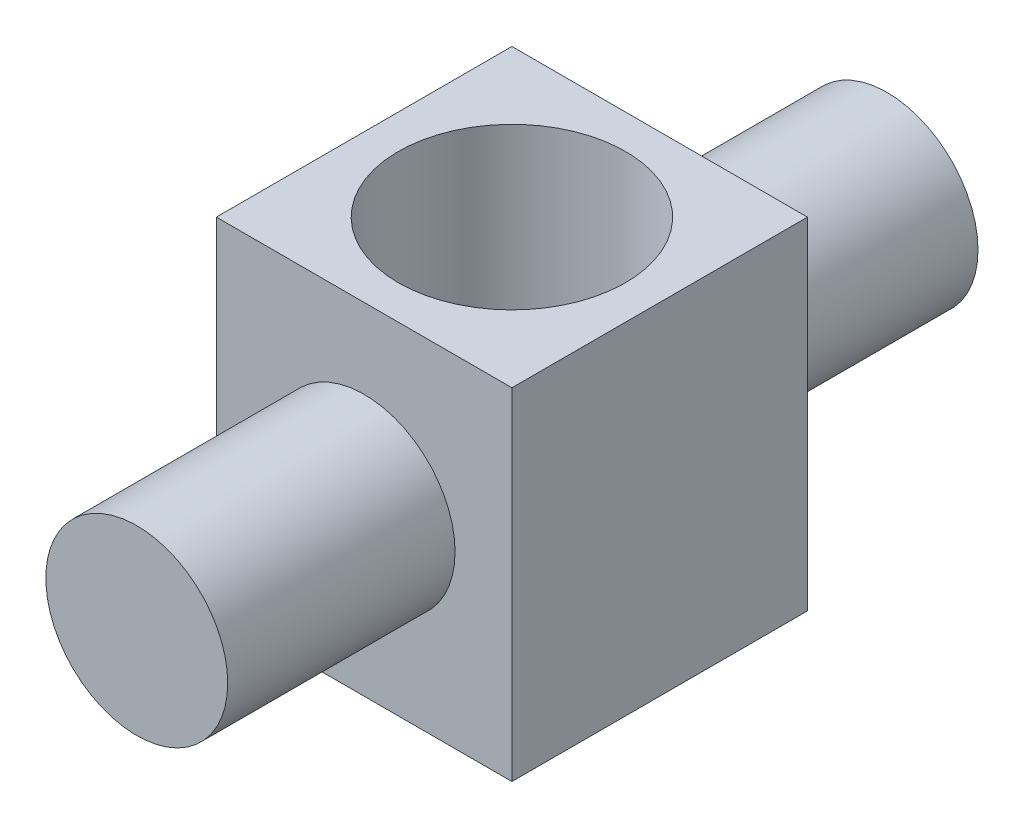
from build123d import *

# Parameters (mm, degrees)
SKETCH1_W           = 13
SKETCH1_H           = 13
SKETCH1_R           = 5
BOSS_EXTRUDE1_DEPTH = 7.5
SKETCH2_R           = 4
BOSS_EXTRUDE2_DEPTH = 10


with BuildPart() as part:
    # Sketch1 → Boss-Extrude1 (new, symmetric)
    with BuildSketch(Plane(origin=(0, 0, 0), x_dir=(1, 0, 0), z_dir=(0, 1, 0))):
        Rectangle(SKETCH1_W, SKETCH1_H)
        with Locations(Location((0, 0, 0), (0, 0, 270))):
            Circle(SKETCH1_R, mode=Mode.SUBTRACT)
    extrude(amount=BOSS_EXTRUDE1_DEPTH, both=True)

    # Sketch2 → Boss-Extrude2 (add)
    with BuildSketch(Plane.XY.offset(6.5)):
        Circle(SKETCH2_R)
    boss_extrude2 = extrude(amount=BOSS_EXTRUDE2_DEPTH)

    # Mirror1: Boss-Extrude2 across plane
    add(boss_extrude2.mirror(Plane.XY))


solid = part.part
